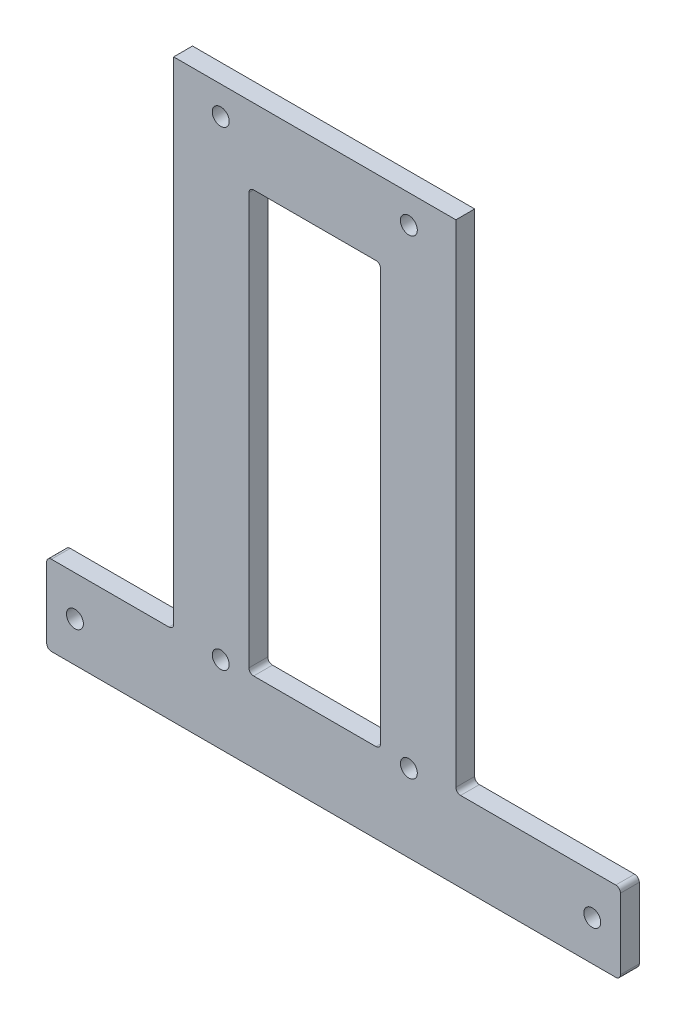
from build123d import *

# Parameters (mm, degrees)
SKETCH1_R           = 9
BOSS_EXTRUDE1_DEPTH = 20


with BuildPart() as part:
    # Sketch1 → Boss-Extrude1 (new body)
    with BuildSketch(Plane.XY):
        with BuildLine():
            Line((5, 0), (605, 0))
            ThreePointArc((605, 0), (608.535533906, 1.464466094), (610, 5))
            Line((610, 5), (610, 80))
            ThreePointArc((610, 80), (608.535533906, 83.535533906), (605, 85))
            Line((605, 85), (440, 85))
            ThreePointArc((440, 85), (436.464466094, 86.464466094), (435, 90))
            Line((435, 90), (435, 612.5))
            Line((435, 612.5), (135, 612.5))
            Line((135, 612.5), (135, 90))
            ThreePointArc((135, 90), (133.535533906, 86.464466094), (130, 85))
            Line((130, 85), (5, 85))
            ThreePointArc((5, 85), (1.464466094, 83.535533906), (0, 80))
            Line((0, 80), (0, 5))
            ThreePointArc((0, 5), (1.464466094, 1.464466094), (5, 0))
        make_face()
        with Locations((30, 42.5)):
            Circle(SKETCH1_R, mode=Mode.SUBTRACT)
        with Locations((580, 42.5)):
            Circle(SKETCH1_R, mode=Mode.SUBTRACT)
        with Locations((185, 582.5)):
            Circle(SKETCH1_R, mode=Mode.SUBTRACT)
        with Locations((385, 582.5)):
            Circle(SKETCH1_R, mode=Mode.SUBTRACT)
        with Locations((185, 82.5)):
            Circle(SKETCH1_R, mode=Mode.SUBTRACT)
        with Locations((385, 82.5)):
            Circle(SKETCH1_R, mode=Mode.SUBTRACT)
        with BuildLine():
            Line((220, 85), (350, 85))
            ThreePointArc((350, 85), (353.535533906, 86.464466094), (355, 90))
            Line((355, 90), (355, 527.5))
            ThreePointArc((355, 527.5), (353.535533906, 531.035533906), (350, 532.5))
            Line((350, 532.5), (220, 532.5))
            ThreePointArc((220, 532.5), (216.464466094, 531.035533906), (215, 527.5))
            Line((215, 527.5), (215, 90))
            ThreePointArc((215, 90), (216.464466094, 86.464466094), (220, 85))
        make_face(mode=Mode.SUBTRACT)
    extrude(amount=BOSS_EXTRUDE1_DEPTH)


solid = part.part
